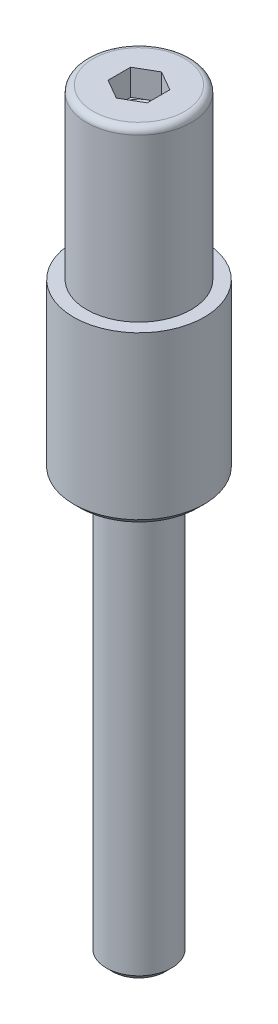
from build123d import *

# Parameters (mm, degrees)
CUT_EXTRUDE_1_DEPTH      = 2
CUT_EXTRUDE_1_DEPTH_BACK = 2


with BuildPart() as part:
    # 草图1 → 旋转1 (revolve)
    with BuildSketch(Plane.XY, mode=Mode.PRIVATE) as revolve_1_sk:
        with BuildLine():
            Line((0, 25.8), (3.5, 25.8))
            ThreePointArc((3.5, 25.8), (3.853553391, 25.653553391), (4, 25.3))
            Line((4, 25.3), (4, 12.9))
            Line((4, 12.9), (5, 12.9))
            Line((5, 12.9), (5, 0.5))
            Line((5, 0.5), (4.5, 0))
            Line((4.5, 0), (2.5, 0))
            Line((2.5, 0), (2.5, -31.5095))
            Line((2.5, -31.5095), (2.0095, -32))
            Line((2.0095, -32), (0, -32))
            Line((0, -32), (0, 25.8))
        make_face()
    revolve(revolve_1_sk.sketch.rotate(Axis((0, -32, 0), (0, 1, 0)), 270), axis=Axis((0, -32, 0), (0, 1, 0)))

    # 草图2 → 切除-拉伸1 (cut, two sides: drawn at the far end of the back side and taken through both)
    with BuildSketch(Plane(origin=(0, 25.8, 0), x_dir=(-1, 0, 0), z_dir=(0, 1, 0)).offset(-CUT_EXTRUDE_1_DEPTH_BACK)):
        Polygon((1.5, -0.866025404), (1.5, 0.866025404), (0, 1.732050808), (-1.5, 0.866025404), (-1.5, -0.866025404), (0, -1.732050808), align=None)
    extrude(amount=CUT_EXTRUDE_1_DEPTH + CUT_EXTRUDE_1_DEPTH_BACK, mode=Mode.SUBTRACT)

    # 草图3 → 切除-旋转1 (revolve, cut)
    with BuildSketch(Plane.XY, mode=Mode.PRIVATE) as cut_revolve_1_sk:
        Polygon((0, 25.8), (1.5, 25.8), (1.5, 23.8), (0, 22.933974596), align=None)
    revolve(cut_revolve_1_sk.sketch.rotate(Axis((0, 22.933974596, 0), (0, 1, 0)), 270), axis=Axis((0, 22.933974596, 0), (0, 1, 0)), mode=Mode.SUBTRACT)


solid = part.part
